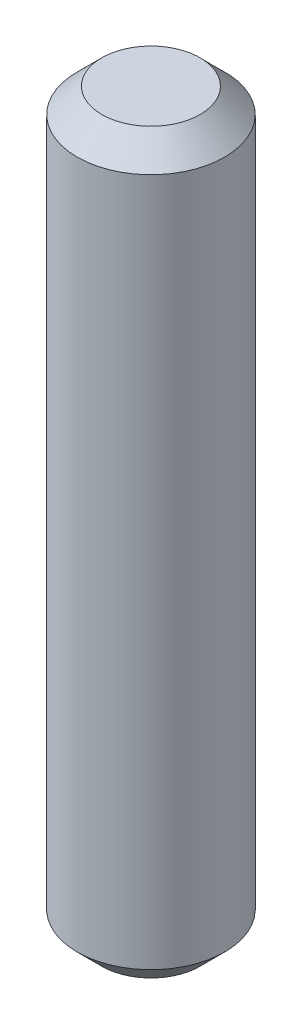
from build123d import *

# Parameters (mm, degrees)
SKETCH1_R           = 1.5
BOSS_EXTRUDE1_DEPTH = 15
CHAMFER1_SIZE       = 0.5


with BuildPart() as part:
    # Sketch1 → Boss-Extrude1 (new body)
    with BuildSketch(Plane(origin=(0, 0, 0), x_dir=(1, 0, 0), z_dir=(0, 1, 0))):
        with Locations(Location((0, 0, 0), (0, 0, 270))):
            Circle(SKETCH1_R)
    extrude(amount=BOSS_EXTRUDE1_DEPTH)

    # Chamfer1
    chamfer1_edges = [part.edges().sort_by_distance(p)[0] for p in [
        (0, 0, -1.5),
        (0, 15, -1.5),
    ]]
    chamfer(chamfer1_edges, length=CHAMFER1_SIZE)


solid = part.part
